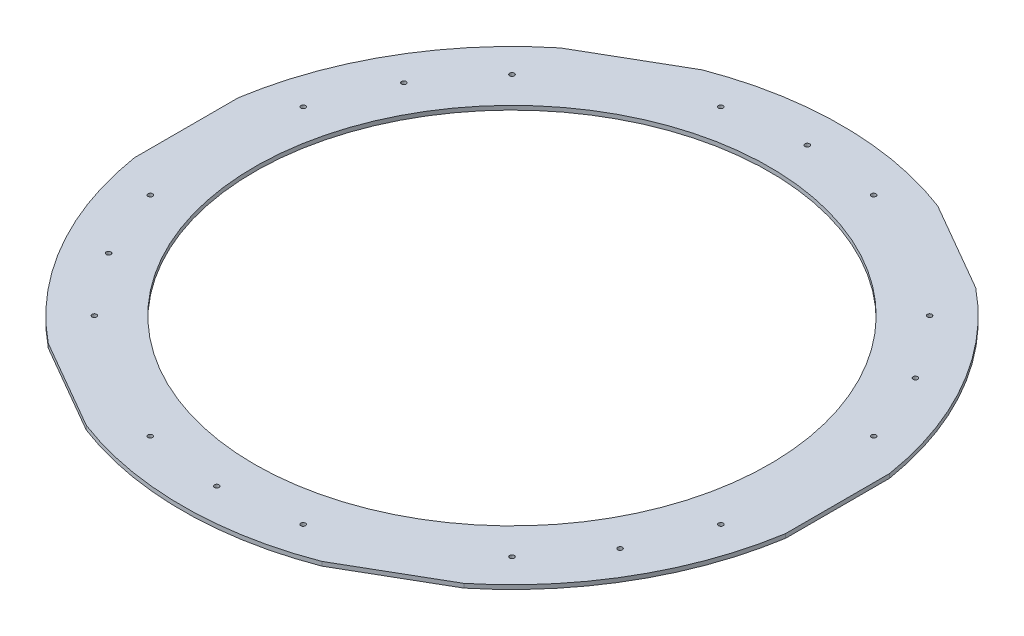
from build123d import *

# Parameters (mm, degrees)
SKETCH1_R             = 480
SKETCH1_R_2           = 375
BOSS_EXTRUDE1_DEPTH   = 6
CUT_EXTRUDE3_REACH    = 680.849
SKETCH2_W             = 12
SKETCH2_H             = 500
CIRPATTERN1_COUNT     = 3
M8_TAPPED_HOLE1_D     = 6.8
M8_TAPPED_HOLE1_DEPTH = 6


with BuildPart() as part:
    # Sketch1 → Boss-Extrude1 (new body)
    with BuildSketch(Plane(origin=(0, 0, 0), x_dir=(1, 0, 0), z_dir=(0, 1, 0))):
        with Locations(Location((0, 0, 0), (0, 0, 270))):
            Circle(SKETCH1_R)
        with Locations(Location((0, 0, 0), (0, 0, 270))):
            Circle(SKETCH1_R_2, mode=Mode.SUBTRACT)
    extrude(amount=BOSS_EXTRUDE1_DEPTH)

    # Sketch2 → Cut-Extrude3 (cut, up to next)
    with BuildSketch(Plane(origin=(0, 0, 0), x_dir=(1, 0, 0), z_dir=(0, 1, 0)), mode=Mode.PRIVATE) as cut_extrude3_sk1:
        with Locations((-480, 0)):
            Rectangle(SKETCH2_W, SKETCH2_H)
    cut_extrude3_tool1 = extrude(cut_extrude3_sk1.sketch, amount=CUT_EXTRUDE3_REACH, mode=Mode.PRIVATE) & part.part
    # Sketch2 → Cut-Extrude3 (cut, up to next)
    with BuildSketch(Plane(origin=(0, 0, 0), x_dir=(1, 0, 0), z_dir=(0, 1, 0)), mode=Mode.PRIVATE) as cut_extrude3_sk2:
        with Locations((480, 0)):
            Rectangle(SKETCH2_W, SKETCH2_H)
    cut_extrude3_tool2 = extrude(cut_extrude3_sk2.sketch, amount=CUT_EXTRUDE3_REACH, mode=Mode.PRIVATE) & part.part
    cut_extrude3_1 = cut_extrude3_tool1.solids().sort_by_distance((-480, 0, 0))[0]
    add(cut_extrude3_1, mode=Mode.SUBTRACT)
    cut_extrude3_2 = cut_extrude3_tool2.solids().sort_by_distance((480, 0, 0))[0]
    add(cut_extrude3_2, mode=Mode.SUBTRACT)
    cut_extrude3 = cut_extrude3_1 + cut_extrude3_2  # Cut-Extrude3 as one shape, for the pattern or mirror that repeats it

    # CirPattern1: Cut-Extrude3 ×3 about axis
    cirpattern1_axis = Axis((0, 0, 0), (0, 1, 0))
    for i in range(1, CIRPATTERN1_COUNT):
        add(cut_extrude3.rotate(cirpattern1_axis, i * 360 / CIRPATTERN1_COUNT), mode=Mode.SUBTRACT)

    # M8 Tapped Hole1
    with Locations(Plane(origin=(0, 6, 0), x_dir=(1, 0, 0), z_dir=(0, 1, 0))):
        with Locations((0, 430), (111.292189394, 415.348105304), (-111.292189394, 415.348105304), (372.390923627, 215), (415.348105304, 111.292189394), (304.05591591, 304.05591591), (372.390923627, -215), (304.05591591, -304.05591591), (415.348105304, -111.292189394), (0, -430), (-111.292189394, -415.348105304), (111.292189394, -415.348105304), (-372.390923627, -215), (-415.348105304, -111.292189394), (-304.05591591, -304.05591591), (-372.390923627, 215), (-304.05591591, 304.05591591), (-415.348105304, 111.292189394), (0, 0)):
            Hole(M8_TAPPED_HOLE1_D / 2, depth=M8_TAPPED_HOLE1_DEPTH)


solid = part.part
